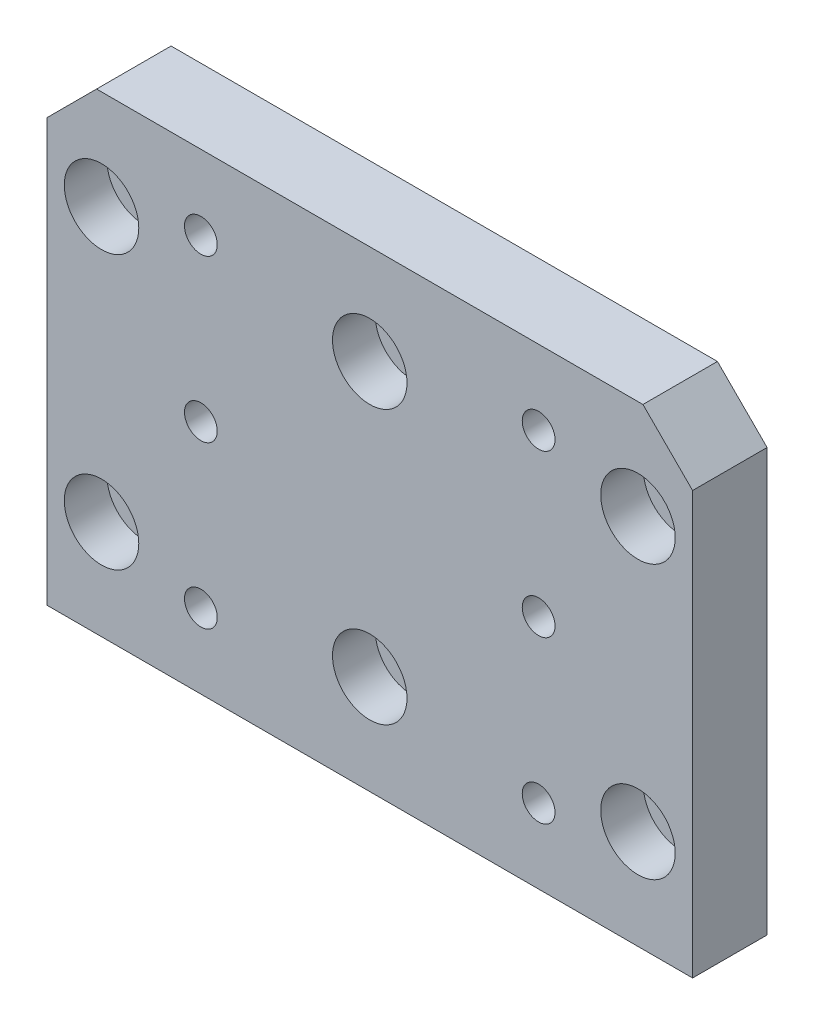
from build123d import *

# Parameters (mm, degrees)
SKETCH1_W                                           = 130
SKETCH1_H                                           = 95
BOSS_EXTRUDE1_DEPTH                                 = 15
CBORE_FOR_M8_HEX_SOCKET_HEAD_CAP_SCREW1_D           = 9
CBORE_FOR_M8_HEX_SOCKET_HEAD_CAP_SCREW1_CBORE_D     = 15
CBORE_FOR_M8_HEX_SOCKET_HEAD_CAP_SCREW1_CBORE_DEPTH = 8.6
CHAMFER1_SIZE                                       = 10
CBORE_FOR_M6_HEX_SOCKET_HEAD_CAP_SCREW1_D           = 6.6
CBORE_FOR_M6_HEX_SOCKET_HEAD_CAP_SCREW1_CBORE_D     = 11
CBORE_FOR_M6_HEX_SOCKET_HEAD_CAP_SCREW1_CBORE_DEPTH = 6.4


with BuildPart() as part:
    # Sketch1 → Boss-Extrude1 (new body)
    with BuildSketch(Plane.XY):
        Rectangle(SKETCH1_W, SKETCH1_H)
    extrude(amount=BOSS_EXTRUDE1_DEPTH)

    # CBORE for M8 Hex Socket Head Cap Screw1 (through all)
    with Locations(Plane.XY.offset(15)):
        with Locations((54, 27.5), (54, -27.5), (-54, 27.5), (-54, -27.5), (0, 27.5), (0, -27.5)):
            CounterBoreHole(CBORE_FOR_M8_HEX_SOCKET_HEAD_CAP_SCREW1_D / 2, CBORE_FOR_M8_HEX_SOCKET_HEAD_CAP_SCREW1_CBORE_D / 2, CBORE_FOR_M8_HEX_SOCKET_HEAD_CAP_SCREW1_CBORE_DEPTH)

    # Chamfer1
    chamfer1_edges = [part.edges().sort_by_distance(p)[0] for p in [
        (-65, 47.5, 7.5),
        (65, 47.5, 7.5),
    ]]
    chamfer(chamfer1_edges, length=CHAMFER1_SIZE)

    # CBORE for M6 Hex Socket Head Cap Screw1 (through all)
    with Locations(Plane(origin=(0, 0, 0), x_dir=(-1, 0, 0), z_dir=(0, 0, -1))):
        with Locations((-34, -32.5), (-34, 0), (-34, 32.5), (34, -32.5), (34, 0), (34, 32.5)):
            CounterBoreHole(CBORE_FOR_M6_HEX_SOCKET_HEAD_CAP_SCREW1_D / 2, CBORE_FOR_M6_HEX_SOCKET_HEAD_CAP_SCREW1_CBORE_D / 2, CBORE_FOR_M6_HEX_SOCKET_HEAD_CAP_SCREW1_CBORE_DEPTH)


solid = part.part
